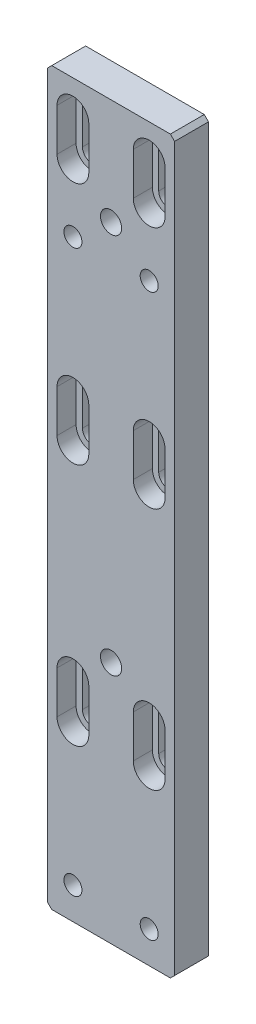
from build123d import *

# Parameters (mm, degrees)
SKETCH_1_W                = 60
SKETCH_1_H                = 345
EXTRUDE_1_DEPTH           = 16
HOLE_WIZARD_1_D           = 9
HOLE_WIZARD_1_CBORE_D     = 15
HOLE_WIZARD_1_CBORE_DEPTH = 9
CHAMFER_1_SIZE            = 2
CUT_EXTRUDE_3_DEPTH       = 9
CUT_EXTRUDE_4_DEPTH       = 176.320420944
HOLE_WIZARD_M10_1_D       = 8.5
HOLE_WIZARD_M10_1_DEPTH   = 27.5
HOLE_WIZARD_M10_1_TIP     = 2.553657631
MM_1_D                    = 10
MM_1_DEPTH                = 25
MM_1_TIP                  = 3.004303095


with BuildPart() as part:
    # 草图1 → 凸台-拉伸1 (new body)
    with BuildSketch(Plane.XY):
        Rectangle(SKETCH_1_W, SKETCH_1_H)
    extrude(amount=EXTRUDE_1_DEPTH)

    # 打孔尺寸(%根据)内六角圆柱头螺钉的类型1 (through all)
    with Locations(Plane.XY.offset(16)):
        with Locations((18, 147.5), (-18, -82.5), (-18, 147.5), (18, -82.5), (-18, 32.5), (18, 32.5)):
            CounterBoreHole(HOLE_WIZARD_1_D / 2, HOLE_WIZARD_1_CBORE_D / 2, HOLE_WIZARD_1_CBORE_DEPTH)

    # 倒角1
    chamfer_1_edges = [part.edges().sort_by_distance(p)[0] for p in [
        (30, -172.5, 8),
        (-30, -172.5, 8),
        (-30, 172.5, 8),
        (30, 172.5, 8),
    ]]
    chamfer(chamfer_1_edges, length=CHAMFER_1_SIZE)

    # 草图7 → 切除-拉伸3 (cut)
    with BuildSketch(Plane.XY.offset(16)):
        with BuildLine():
            Line((-10.5, 157.5), (-10.5, 137.5))
            ThreePointArc((-10.5, 137.5), (-18, 130), (-25.5, 137.5))
            Line((-25.5, 137.5), (-25.5, 157.5))
            ThreePointArc((-25.5, 157.5), (-18, 165), (-10.5, 157.5))
        make_face()
        with BuildLine():
            Line((25.5, 157.5), (25.5, 137.5))
            ThreePointArc((25.5, 137.5), (18, 130), (10.5, 137.5))
            Line((10.5, 137.5), (10.5, 157.5))
            ThreePointArc((10.5, 157.5), (18, 165), (25.5, 157.5))
        make_face()
        with BuildLine():
            Line((-25.5, 22.5), (-25.5, 42.5))
            ThreePointArc((-25.5, 42.5), (-18, 50), (-10.5, 42.5))
            Line((-10.5, 42.5), (-10.5, 22.5))
            ThreePointArc((-10.5, 22.5), (-18, 15), (-25.5, 22.5))
        make_face()
        with BuildLine():
            Line((10.5, 22.5), (10.5, 42.5))
            ThreePointArc((10.5, 42.5), (18, 50), (25.5, 42.5))
            Line((25.5, 42.5), (25.5, 22.5))
            ThreePointArc((25.5, 22.5), (18, 15), (10.5, 22.5))
        make_face()
        with BuildLine():
            Line((-25.5, -92.5), (-25.5, -72.5))
            ThreePointArc((-25.5, -72.5), (-18, -65), (-10.5, -72.5))
            Line((-10.5, -72.5), (-10.5, -92.5))
            ThreePointArc((-10.5, -92.5), (-18, -100), (-25.5, -92.5))
        make_face()
        with BuildLine():
            Line((10.5, -92.5), (10.5, -72.5))
            ThreePointArc((10.5, -72.5), (18, -65), (25.5, -72.5))
            Line((25.5, -72.5), (25.5, -92.5))
            ThreePointArc((25.5, -92.5), (18, -100), (10.5, -92.5))
        make_face()
    extrude(amount=-CUT_EXTRUDE_3_DEPTH, mode=Mode.SUBTRACT)

    # 草图8 → 切除-拉伸4 (cut, through all)
    with BuildSketch(Plane.XY.offset(7)):
        with BuildLine():
            Line((-22.5, 137.5), (-22.5, 157.5))
            ThreePointArc((-22.5, 157.5), (-18, 162), (-13.5, 157.5))
            Line((-13.5, 157.5), (-13.5, 137.5))
            ThreePointArc((-13.5, 137.5), (-18, 133), (-22.5, 137.5))
        make_face()
        with BuildLine():
            Line((13.5, 137.5), (13.5, 157.5))
            ThreePointArc((13.5, 157.5), (18, 162), (22.5, 157.5))
            Line((22.5, 157.5), (22.5, 137.5))
            ThreePointArc((22.5, 137.5), (18, 133), (13.5, 137.5))
        make_face()
        with BuildLine():
            Line((-22.5, 22.5), (-22.5, 42.5))
            ThreePointArc((-22.5, 42.5), (-18, 47), (-13.5, 42.5))
            Line((-13.5, 42.5), (-13.5, 22.5))
            ThreePointArc((-13.5, 22.5), (-18, 18), (-22.5, 22.5))
        make_face()
        with BuildLine():
            Line((13.5, 22.5), (13.5, 42.5))
            ThreePointArc((13.5, 42.5), (18, 47), (22.5, 42.5))
            Line((22.5, 42.5), (22.5, 22.5))
            ThreePointArc((22.5, 22.5), (18, 18), (13.5, 22.5))
        make_face()
        with BuildLine():
            Line((-22.5, -92.5), (-22.5, -72.5))
            ThreePointArc((-22.5, -72.5), (-18, -68), (-13.5, -72.5))
            Line((-13.5, -72.5), (-13.5, -92.5))
            ThreePointArc((-13.5, -92.5), (-18, -97), (-22.5, -92.5))
        make_face()
        with BuildLine():
            Line((13.5, -92.5), (13.5, -72.5))
            ThreePointArc((13.5, -72.5), (18, -68), (22.5, -72.5))
            Line((22.5, -72.5), (22.5, -92.5))
            ThreePointArc((22.5, -92.5), (18, -97), (13.5, -92.5))
        make_face()
    extrude(amount=-CUT_EXTRUDE_4_DEPTH, mode=Mode.SUBTRACT)

    # M10 螺纹孔1
    with Locations(Plane.XY.offset(16)):
        with Locations((-18, 107.5), (18, 107.5), (-18, -157.5), (18, -157.5)):
            Hole(HOLE_WIZARD_M10_1_D / 2, depth=HOLE_WIZARD_M10_1_DEPTH)
            with Locations((0, 0, -(HOLE_WIZARD_M10_1_DEPTH + HOLE_WIZARD_M10_1_TIP / 2))):  # 118° drill point
                Cone(0, HOLE_WIZARD_M10_1_D / 2, HOLE_WIZARD_M10_1_TIP, mode=Mode.SUBTRACT)

    # 大小mm 暗销孔1
    with Locations(Plane.XY.offset(16)):
        with Locations((0, -57.5), (0, 122.5)):
            Hole(MM_1_D / 2, depth=MM_1_DEPTH)
            with Locations((0, 0, -(MM_1_DEPTH + MM_1_TIP / 2))):  # 118° drill point
                Cone(0, MM_1_D / 2, MM_1_TIP, mode=Mode.SUBTRACT)


solid = part.part
